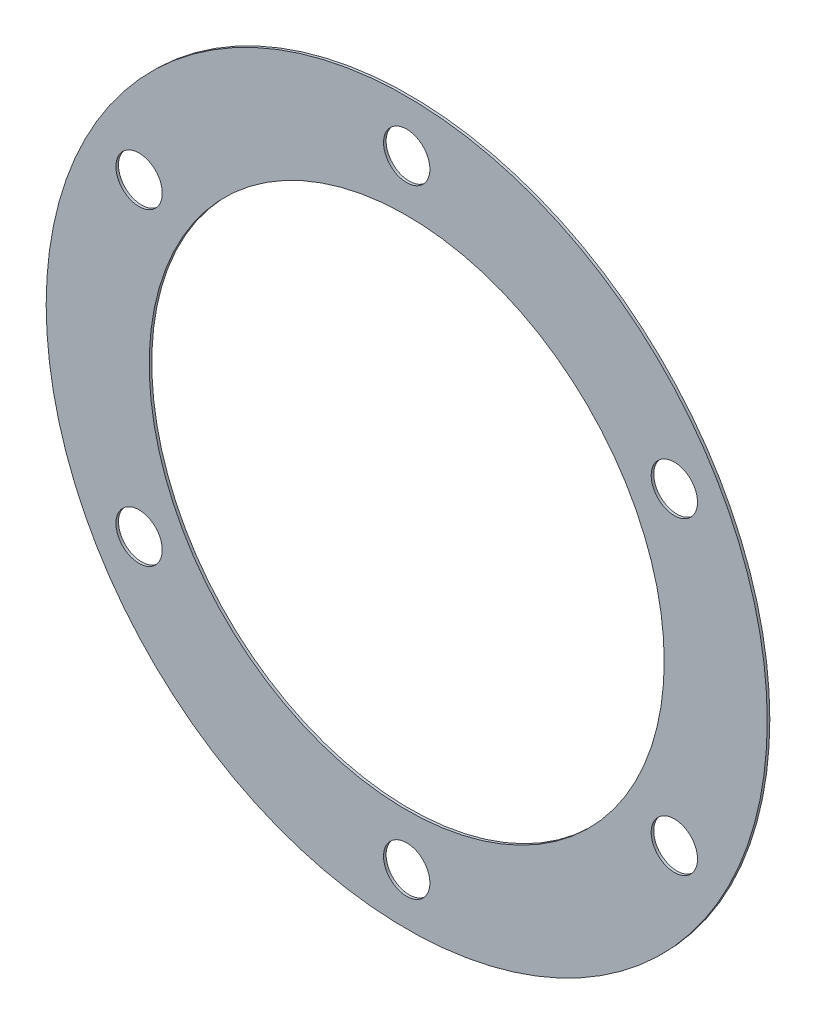
from build123d import *

# Parameters (mm, degrees)
SKETCH1_R           = 70
SKETCH1_R_2         = 50
BOSS_EXTRUDE1_DEPTH = 0.5
SKETCH2_R           = 4.5
CUT_EXTRUDE1_DEPTH  = 99.996212049
CIRPATTERN1_COUNT   = 6


with BuildPart() as part:
    # Sketch1 → Boss-Extrude1 (new body)
    with BuildSketch(Plane.XY):
        Circle(SKETCH1_R)
        Circle(SKETCH1_R_2, mode=Mode.SUBTRACT)
    extrude(amount=BOSS_EXTRUDE1_DEPTH)

    # Sketch2 → Cut-Extrude1 (cut, through all)
    with BuildSketch(Plane.XY.offset(0.5)):
        with Locations((0, 60)):
            Circle(SKETCH2_R)
    cut_extrude1 = extrude(amount=-CUT_EXTRUDE1_DEPTH, mode=Mode.SUBTRACT)

    # CirPattern1: Cut-Extrude1 ×6 about axis
    cirpattern1_axis = Axis((0, 0, 0), (0, 0, 1))
    for i in range(1, CIRPATTERN1_COUNT):
        add(cut_extrude1.rotate(cirpattern1_axis, i * 360 / CIRPATTERN1_COUNT), mode=Mode.SUBTRACT)


solid = part.part
